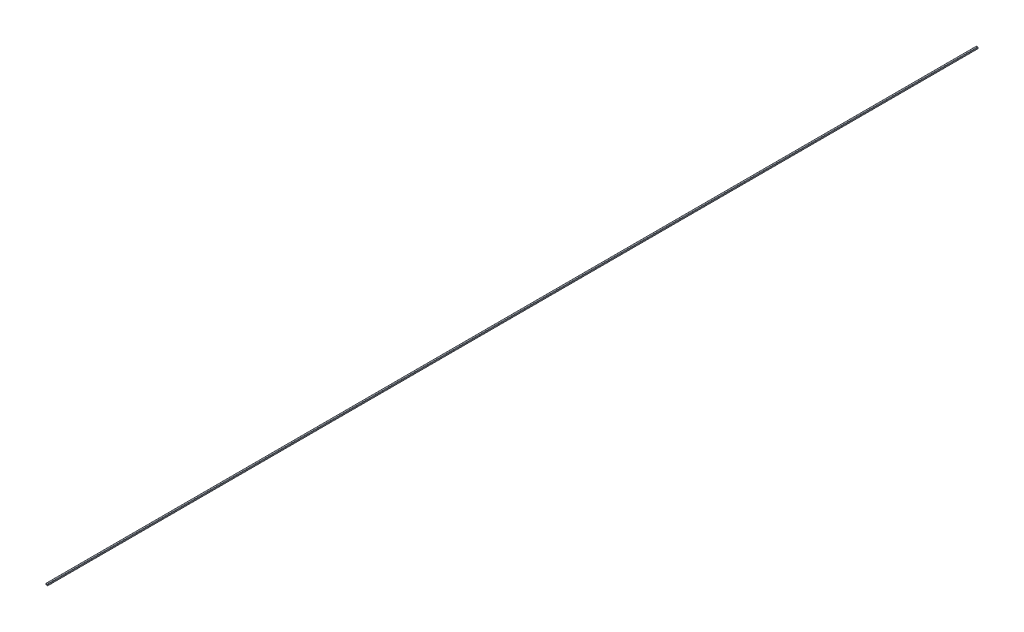
SolidWorks part; units mm, degrees
ref_plane "Front Plane" through (0, 0, 0) normal (0, 0, 1) x (1, 0, 0)
ref_plane "Top Plane" through (0, 0, 0) normal (0, 1, 0) x (1, 0, 0)
ref_plane "Right Plane" through (0, 0, 0) normal (1, 0, 0) x (0, 0, -1)
other "Configuration Table"
sketch "Sketch1" plane through (0, 0, 0) normal (0, 0, 1) x (1, 0, 0)
  line L0 (-10, -13.2) -> (-6.5, -13.2)
  line L1 (-10, 15) -> (10, 15)
  line L2 (-16, 9) -> (-16, -9)
  line L3 (-10, -15) -> (-6.5, -15)
  line L4 (16, 9) -> (16, -9)
  line L5 (-16, 15) -> (16, -15) construction
  line L6 (-16, -15) -> (16, 15) construction
  line L7 (-14.2, 9) -> (-14.2, -9)
  line L8 (6.5, -15) -> (10, -15)
  line L9 (-10, 13.2) -> (10, 13.2)
  line L10 (14.2, 9) -> (14.2, -9)
  line L11 (6.5, -13.2) -> (10, -13.2)
  line L12 (-6.5, -15) -> (-6.5, -13.2)
  line L13 (6.5, -15) -> (6.5, -13.2)
  arc A0 (-16, -9) -> (-10, -15) centre (-10, -9) ccw
  arc A1 (10, -15) -> (16, -9) centre (10, -9) ccw
  arc A2 (10, 15) -> (16, 9) centre (10, 9) cw
  arc A3 (-10, 15) -> (-16, 9) centre (-10, 9) ccw
  arc A4 (-14.2, -9) -> (-10, -13.2) centre (-10, -9) ccw
  arc A5 (-10, 13.2) -> (-14.2, 9) centre (-10, 9) ccw
  arc A6 (10, 13.2) -> (14.2, 9) centre (10, 9) cw
  arc A7 (10, -13.2) -> (14.2, -9) centre (10, -9) ccw
  point P0 (0, 0)
  dimension "D5" = 6
  dimension "D1" = 32
  dimension "D2" = 30
  dimension "D3" = 9.5
  dimension "D4" = 9.5
  dimension "D6" = 1.8
extrude "Boss-Extrude1" add sketch "Sketch1" along normal blind 16840
